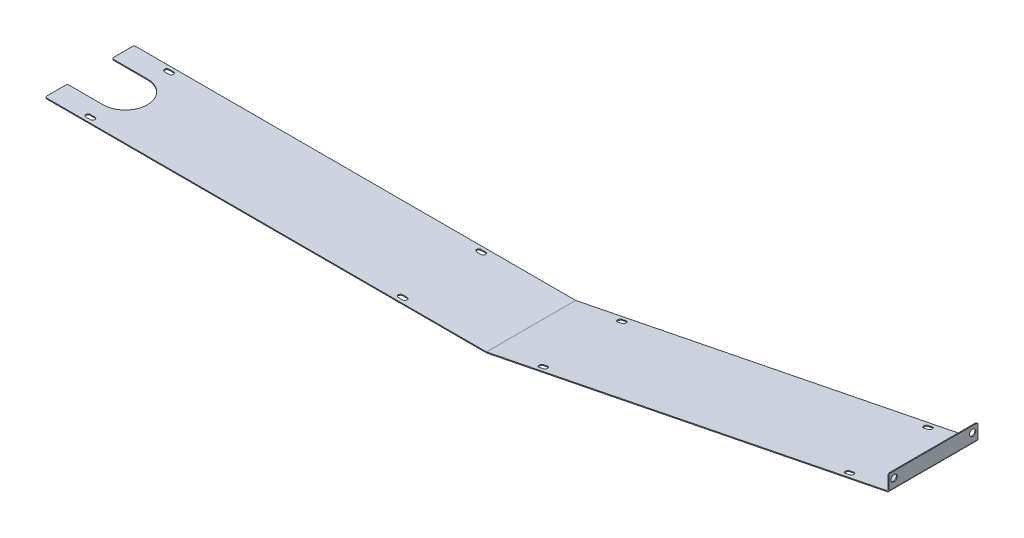
from build123d import *

# Parameters (mm, degrees)
EXTRUDE_THIN1_DEPTH = 50
SKETCH2_R           = 3.5
CUT_EXTRUDE1_DEPTH  = 953.351825745
CUT_EXTRUDE2_DEPTH  = 954.456868453
CUT_EXTRUDE3_DEPTH  = 951.073377733
CUT_EXTRUDE4_DEPTH  = 954.344114158
FILLET1_R           = 2


with BuildPart() as part:
    # Sketch1 → Extrude-Thin1 (new, symmetric)
    with BuildSketch(Plane.XY):
        Polygon((0, 0), (495, 0), (945, 90), (945, 107), (946, 107), (946, 89.180196097), (495.099019514, -1), (0, -1), align=None)
    extrude(amount=EXTRUDE_THIN1_DEPTH, both=True)

    # Sketch2 → Cut-Extrude1 (cut, through all)
    with BuildSketch(Plane.ZY.offset(-945)):
        with Locations((-44, 100)):
            Circle(SKETCH2_R)
        with Locations((44, 100)):
            Circle(SKETCH2_R)
    extrude(amount=-CUT_EXTRUDE1_DEPTH, mode=Mode.SUBTRACT)

    # Sketch3 → Cut-Extrude2 (cut, through all)
    with BuildSketch(Plane.XZ.offset(1)):
        with BuildLine():
            Line((42.5, 46.5), (47.5, 46.5))
            ThreePointArc((47.5, 46.5), (50, 44), (47.5, 41.5))
            Line((47.5, 41.5), (42.5, 41.5))
            ThreePointArc((42.5, 41.5), (40, 44), (42.5, 46.5))
        make_face()
        with BuildLine():
            Line((42.5, -41.5), (47.5, -41.5))
            ThreePointArc((47.5, -41.5), (50, -44), (47.5, -46.5))
            Line((47.5, -46.5), (42.5, -46.5))
            ThreePointArc((42.5, -46.5), (40, -44), (42.5, -41.5))
        make_face()
        with BuildLine():
            Line((392.5, -41.5), (397.5, -41.5))
            ThreePointArc((397.5, -41.5), (400, -44), (397.5, -46.5))
            Line((397.5, -46.5), (392.5, -46.5))
            ThreePointArc((392.5, -46.5), (390, -44), (392.5, -41.5))
        make_face()
        with BuildLine():
            Line((392.5, 46.5), (397.5, 46.5))
            ThreePointArc((397.5, 46.5), (400, 44), (397.5, 41.5))
            Line((397.5, 41.5), (392.5, 41.5))
            ThreePointArc((392.5, 41.5), (390, 44), (392.5, 46.5))
        make_face()
    extrude(amount=-CUT_EXTRUDE2_DEPTH, mode=Mode.SUBTRACT)

    # Sketch4 → Cut-Extrude3 (cut, through all)
    with BuildSketch(Plane(origin=(19.038461538, -95.192307692, 0), x_dir=(0.9805806756909202, 0.1961161351381841, 0), z_dir=(-0.1961161351381841, 0.9805806756909202, 0))):
        with BuildLine():
            Line((541.79919069, 46.5), (546.79919069, 46.5))
            ThreePointArc((546.79919069, 46.5), (549.29919069, 44), (546.79919069, 41.5))
            Line((546.79919069, 41.5), (541.79919069, 41.5))
            ThreePointArc((541.79919069, 41.5), (539.29919069, 44), (541.79919069, 46.5))
        make_face()
        with BuildLine():
            Line((541.79919069, -41.5), (546.79919069, -41.5))
            ThreePointArc((546.79919069, -41.5), (549.29919069, -44), (546.79919069, -46.5))
            Line((546.79919069, -46.5), (541.79919069, -46.5))
            ThreePointArc((541.79919069, -46.5), (539.29919069, -44), (541.79919069, -41.5))
        make_face()
        with BuildLine():
            Line((891.79919069, -41.5), (896.79919069, -41.5))
            ThreePointArc((896.79919069, -41.5), (899.29919069, -44), (896.79919069, -46.5))
            Line((896.79919069, -46.5), (891.79919069, -46.5))
            ThreePointArc((891.79919069, -46.5), (889.29919069, -44), (891.79919069, -41.5))
        make_face()
        with BuildLine():
            Line((891.79919069, 46.5), (896.79919069, 46.5))
            ThreePointArc((896.79919069, 46.5), (899.29919069, 44), (896.79919069, 41.5))
            Line((896.79919069, 41.5), (891.79919069, 41.5))
            ThreePointArc((891.79919069, 41.5), (889.29919069, 44), (891.79919069, 46.5))
        make_face()
    extrude(amount=-CUT_EXTRUDE3_DEPTH, mode=Mode.SUBTRACT)

    # Sketch5 → Cut-Extrude4 (cut, through all)
    with BuildSketch(Plane(origin=(0, 0, 0), x_dir=(1, 0, 0), z_dir=(0, 1, 0))):
        with BuildLine():
            Line((0, -25), (40, -25))
            ThreePointArc((40, -25), (65, 0), (40, 25))
            Line((40, 25), (0, 25))
            Line((0, 25), (0, -25))
        make_face()
    extrude(amount=-CUT_EXTRUDE4_DEPTH, mode=Mode.SUBTRACT)

    # Fillet1
    fillet1_edges = [part.edges().sort_by_distance(p)[0] for p in [
        (946, 89.180196097, 0),
        (495.099019514, -1, 0),
        (495, 0, 0),
        (945, 90, 0),
        (0, -0.5, 25),
        (0, -0.5, -25),
        (0, -0.5, 50),
        (945.5, 107, 50),
        (0, -0.5, -50),
        (945.5, 107, -50),
    ]]
    fillet(fillet1_edges, radius=FILLET1_R)


solid = part.part
